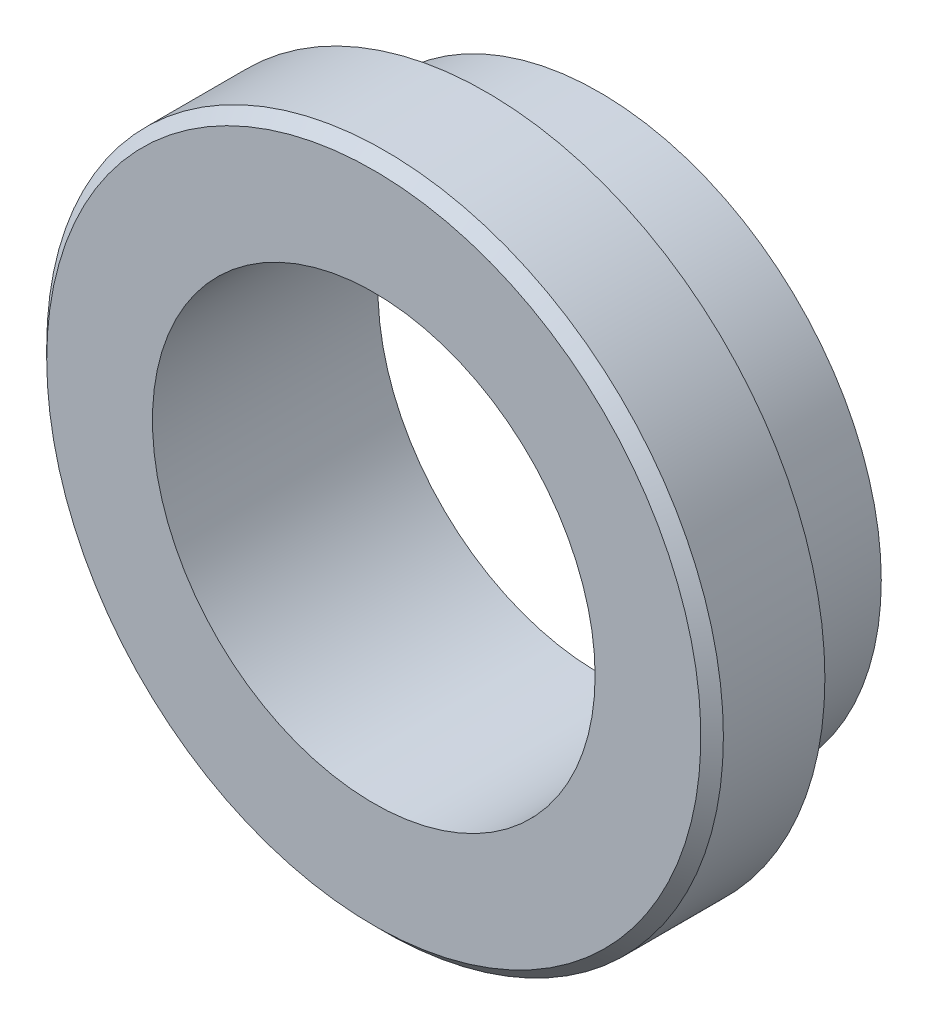
SolidWorks part; units mm, degrees
material "45#调质"
ref_plane "Front Plane" through (0, 0, 0) normal (0, 0, 1) x (1, 0, 0)
ref_plane "Top Plane" through (0, 0, 0) normal (0, 1, 0) x (1, 0, 0)
ref_plane "Right Plane" through (0, 0, 0) normal (1, 0, 0) x (0, 0, -1)
sketch "Sketch1" plane through (0, 0, 0) normal (1, 0, 0) x (0, 0, -1)
  line L0 (0, 0) -> (0, 25)
  line L1 (0, 25) -> (-10, 25)
  line L2 (-10, 25) -> (-10, 30)
  line L3 (-10, 30) -> (-20, 30)
  line L4 (-20, 30) -> (-20, 0)
  line L5 (-20, 0) -> (0, 0)
  dimension "D1" = 25
  dimension "D2" = 5
  dimension "D3" = 10
  dimension "D4" = 10
revolve "Revolve1" add sketch "Sketch1" angle 360 about L5
hole_wizard "G1-1/4 Tapped Hole1" positions "Sketch2" profile "Sketch3" tap size "G1-1/4" standard "GB" end condition through all
sketch "Sketch2" plane through (0, 0, 20) normal (0, 0, 1) x (1, 0, 0)
  point P0 (0, 0)
sketch "Sketch3" plane through (0, 0, 20) normal (1, 0, 0) x (0, -1, 0)
  line L0 (0, 0) -> (0, 20)
  line L1 (0, 20) -> (19.625, 20)
  line L2 (19.625, 20) -> (19.625, 0)
  line L5 (19.625, 0) -> (0, 0)
  line L11 (0, -6.35) -> (0, 107.95) construction
  dimension "通孔螺纹孔钻头直径" = 39.25
  dimension "通孔螺纹孔钻头深度" = 20
cosmetic thread "Cosmetic thread1" parameters "D2"=41.91
chamfer "Chamfer1" distance 1 angle 45 1 edges at (30, 0, 20)
